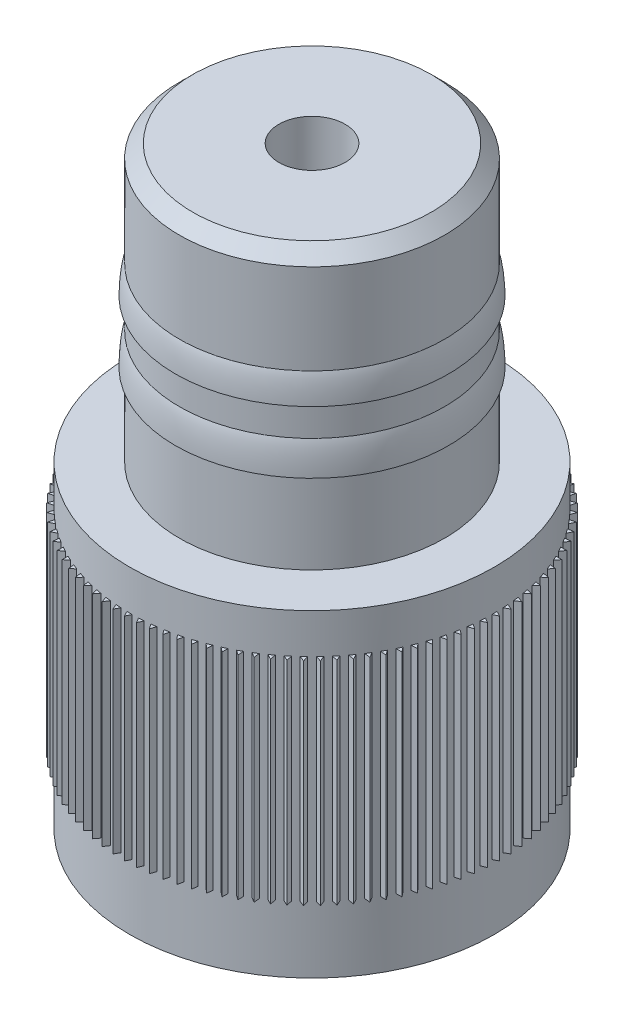
SolidWorks part; units mm, degrees
material "黄铜"
ref_plane "Front Plane" through (0, 0, 0) normal (0, 0, 1) x (1, 0, 0)
ref_plane "Top Plane" through (0, 0, 0) normal (0, 1, 0) x (1, 0, 0)
ref_plane "Right Plane" through (0, 0, 0) normal (1, 0, 0) x (0, 0, -1)
sketch "Sketch1" plane through (0, 0, 0) normal (0, 0, 1) x (1, 0, 0)
  line L0 (0, -30.5763) -> (0, 79.9254) construction
  line L1 (-5, 0) -> (-5, 3.1)
  line L2 (-5, 0) -> (-6.88, 0)
  line L3 (-6.88, 0) -> (-6.88, -12)
  line L4 (-6.88, -12) -> (-3.225, -12)
  line L5 (-1.25, 0) -> (-1.25, 10.4)
  line L6 (-5, 10.4) -> (-1.25, 10.4)
  line L7 (-1.25, 0) -> (-2.525, 0)
  line L8 (-3.225, 0) -> (-3.225, -12)
  line L9 (-5.15, 5.4408) -> (-5, 5.4408)
  line L10 (-2.725, 0) -> (-2.725, -8.44)
  line L11 (-5.15, 3.1) -> (-5, 3.1)
  line L12 (-2.725, -8.44) -> (-2.525, -8.44)
  line L13 (-2.525, -8.44) -> (-2.525, 0)
  line L14 (-2.725, 0) -> (-3.225, 0)
  line L15 (2.2748, 6.5) -> (-3.25, 6.5) construction
  line L16 (-5, 6.5) -> (-5, 10.4)
  line L17 (-5, 4.297) -> (-5, 5.4408)
  spline S5 degree 3 poles (-5, 6.5) (-5.0476, 6.3634) (-5.0815, 6.2026) (-5.1301, 5.8403) (-5.144, 5.6451) (-5.15, 5.4408) knots 0 0 0 0 0.5 0.5 1 1 1 1
  spline S6 degree 3 poles (-5, 4.297) (-5.0512, 4.1421) (-5.0865, 3.9602) (-5.1348, 3.5508) (-5.147, 3.3305) (-5.15, 3.1) knots 0 0 0 0 0.5 0.5 1 1 1 1
  dimension "D1" = 3.1
  dimension "D2" = 13.76
  dimension "D3" = 10
  dimension "D4" = 10.4
  dimension "D5" = 0.15
  dimension "D6" = 12
  dimension "D7" = 6.45
  dimension "D8" = 2.5
  dimension "D9" = 12
  dimension "D10" = 0.2
  dimension "D11" = 0.5
  dimension "D12" = 3.56
revolve "Revolve1" add sketch "Sketch1" angle 360 about L0
chamfer "Chamfer1" distance 0.5 angle 45 1 edges at (0, 10.4, -5)
ref_plane "Plane1" through (0, -9.5, 0) normal (0, -1, 0) x (1, 0, 0)
sketch "Sketch2" plane through (0, -9.5, 0) normal (0, -1, 0) x (1, 0, 0)
  line L0 (0, 0) -> (0, 7.4436) construction
  line L1 (0, 7.08) -> (-0.1, 6.8793)
  line L2 (0, 7.08) -> (0.1, 6.8793)
  circle A1 centre (0, 0) radius 6.88
  arc A2 (0.1, 6.8793) -> (-0.1, 6.8793) centre (0, 0) ccw
  dimension "D2" = 0.2
  dimension "D3" = 0.2
  dimension "D1" = 0
extrude "Boss-Extrude1" add sketch "Sketch2" against normal blind 8
pattern_circular "CirPattern1" count 100 over 360 about axis through (0, 0, 0) along (0, 1, 0) of "Boss-Extrude1"
